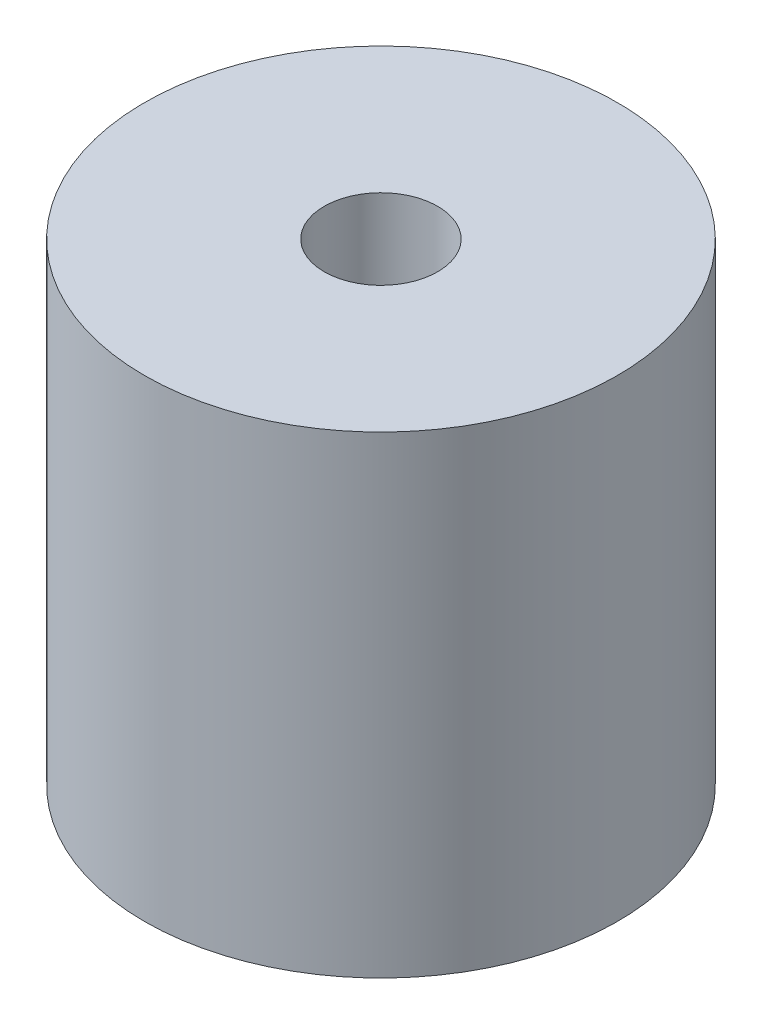
SolidWorks part; units mm, degrees
ref_plane "Front Plane" through (0, 0, 0) normal (0, 0, 1) x (1, 0, 0)
ref_plane "Top Plane" through (0, 0, 0) normal (0, 1, 0) x (1, 0, 0)
ref_plane "Right Plane" through (0, 0, 0) normal (1, 0, 0) x (0, 0, -1)
sketch "Sketch1" plane through (0, 0, 0) normal (0, 1, 0) x (1, 0, 0)
  circle A0 centre (0, 0) radius 12.5
  circle A1 centre (0, 0) radius 3
  dimension "D1" = 6
  dimension "D2" = 25
extrude "Boss-Extrude1" add sketch "Sketch1" along normal blind 25
